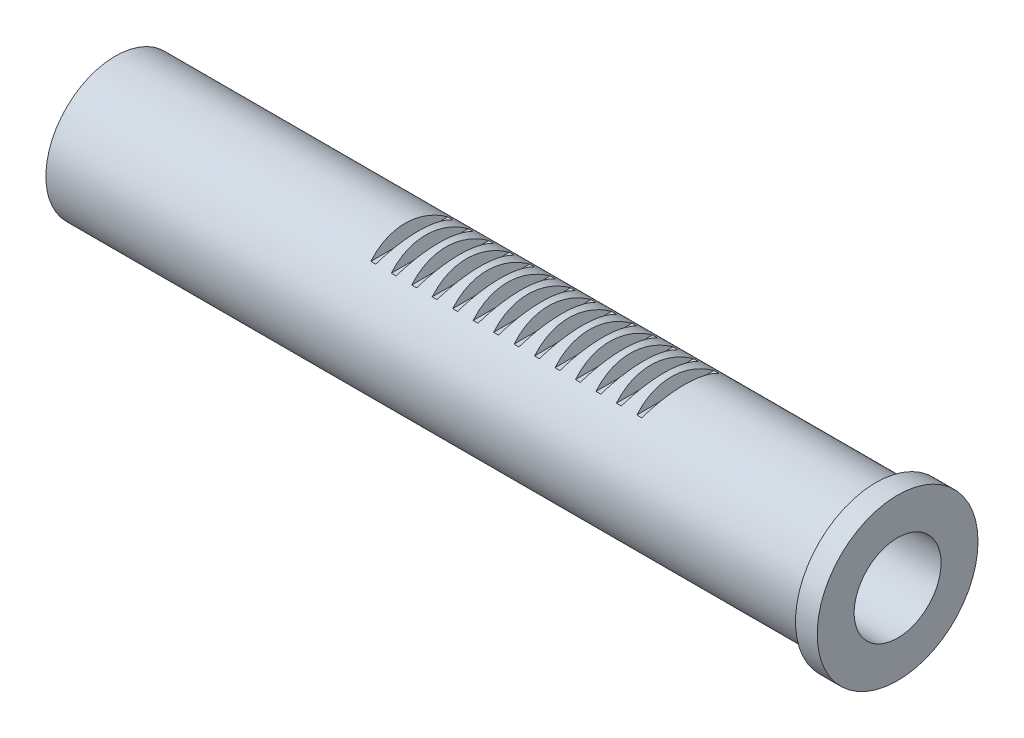
SolidWorks part; units mm, degrees
ref_plane "Front Plane" through (0, 0, 0) normal (0, 0, 1) x (1, 0, 0)
ref_plane "Top Plane" through (0, 0, 0) normal (0, 1, 0) x (1, 0, 0)
ref_plane "Right Plane" through (0, 0, 0) normal (1, 0, 0) x (0, 0, -1)
other "Configuration Table"
sketch "Sketch1" plane through (0, 0, 0) normal (1, 0, 0) x (0, 0, -1)
  circle A0 centre (0, 0) radius 16
  dimension "D1" = 32
extrude "Boss-Extrude1" add sketch "Sketch1" along normal blind 175
sketch "Sketch2" plane through (175, 0, 0) normal (1, 0, 0) x (0, 0, -1)
  circle A0 centre (0, 0) radius 18.5
  dimension "D1" = 37
extrude "Boss-Extrude2" add sketch "Sketch2" along normal blind 5
sketch "Sketch3" plane through (180, 0, 0) normal (1, 0, 0) x (0, 0, -1)
  circle A0 centre (0, 0) radius 10
  dimension "D1" = 20
extrude "Cut-Extrude1" cut sketch "Sketch3" against normal blind 100
sketch "Sketch4" plane through (180, 0, 0) normal (1, 0, 0) x (0, 0, -1)
  circle A0 centre (0, 0) radius 6
  dimension "D1" = 12
extrude "Cut-Extrude2" cut sketch "Sketch4" against normal blind 8000
sketch "Sketch5" plane through (0, 0, 0) normal (0, 0, 1) x (1, 0, 0)
  line L0 (0, 0) -> (50, 0)
  line L1 (0, 6) -> (0, -6) construction
  line L2 (50, 0) -> (50, 6)
  line L3 (50, 6) -> (0, 11)
  line L4 (0, 16) -> (0, -16) construction
  line L5 (0, 11) -> (0, 0)
  line L6 (50, 6) -> (47, 6) construction
  line L7 (47, 6) -> (47, 6.3) construction
  line L8 (80, -6) -> (80, 6) construction
  dimension "D1" = 6
  dimension "D2" = 3
  dimension "D3" = 0.3
  dimension "D4" = 30
revolve "Cut-Revolve1" cut sketch "Sketch5" angle 360 about L0
sketch "Sketch6" plane through (0, 0, 0) normal (0, 0, 1) x (1, 0, 0)
  line L0 (0, 0) -> (68.2, 0) construction
  line L1 (68.2, 0) -> (68.2, 41.9266) construction
  line L2 (69.9952, 16.6972) -> (66.4048, 16.6972)
  line L3 (66.4048, 16.6972) -> (67.635, 13.3172)
  line L4 (67.635, 13.3172) -> (68.765, 13.3172)
  line L5 (67.0225, 15) -> (69.3775, 15) construction
  line L6 (180, -18.5) -> (180, 18.5) construction
  line L7 (69.9952, 16.6972) -> (68.765, 13.3172)
  line L8 (72.345, 13.3172) -> (73.475, 13.3172)
  line L9 (74.7052, 16.6972) -> (73.475, 13.3172)
  line L10 (74.7052, 16.6972) -> (71.1148, 16.6972)
  line L11 (71.1148, 16.6972) -> (72.345, 13.3172)
  line L12 (77.055, 13.3172) -> (78.185, 13.3172)
  line L13 (79.4152, 16.6972) -> (78.185, 13.3172)
  line L14 (79.4152, 16.6972) -> (75.8248, 16.6972)
  line L15 (75.8248, 16.6972) -> (77.055, 13.3172)
  line L16 (81.765, 13.3172) -> (82.895, 13.3172)
  line L17 (84.1252, 16.6972) -> (82.895, 13.3172)
  line L18 (84.1252, 16.6972) -> (80.5348, 16.6972)
  line L19 (80.5348, 16.6972) -> (81.765, 13.3172)
  line L20 (86.475, 13.3172) -> (87.605, 13.3172)
  line L21 (88.8352, 16.6972) -> (87.605, 13.3172)
  line L22 (88.8352, 16.6972) -> (85.2448, 16.6972)
  line L23 (85.2448, 16.6972) -> (86.475, 13.3172)
  line L24 (91.185, 13.3172) -> (92.315, 13.3172)
  line L25 (93.5452, 16.6972) -> (92.315, 13.3172)
  line L26 (93.5452, 16.6972) -> (89.9548, 16.6972)
  line L27 (89.9548, 16.6972) -> (91.185, 13.3172)
  line L28 (95.895, 13.3172) -> (97.025, 13.3172)
  line L29 (98.2552, 16.6972) -> (97.025, 13.3172)
  line L30 (98.2552, 16.6972) -> (94.6648, 16.6972)
  line L31 (94.6648, 16.6972) -> (95.895, 13.3172)
  line L32 (100.605, 13.3172) -> (101.735, 13.3172)
  line L33 (102.9652, 16.6972) -> (101.735, 13.3172)
  line L34 (102.9652, 16.6972) -> (99.3748, 16.6972)
  line L35 (99.3748, 16.6972) -> (100.605, 13.3172)
  line L36 (105.315, 13.3172) -> (106.445, 13.3172)
  line L37 (107.6752, 16.6972) -> (106.445, 13.3172)
  line L38 (107.6752, 16.6972) -> (104.0848, 16.6972)
  line L39 (104.0848, 16.6972) -> (105.315, 13.3172)
  line L40 (110.025, 13.3172) -> (111.155, 13.3172)
  line L41 (112.3852, 16.6972) -> (111.155, 13.3172)
  line L42 (112.3852, 16.6972) -> (108.7948, 16.6972)
  line L43 (108.7948, 16.6972) -> (110.025, 13.3172)
  line L44 (114.735, 13.3172) -> (115.865, 13.3172)
  line L45 (117.0952, 16.6972) -> (115.865, 13.3172)
  line L46 (117.0952, 16.6972) -> (113.5048, 16.6972)
  line L47 (113.5048, 16.6972) -> (114.735, 13.3172)
  line L48 (119.445, 13.3172) -> (120.575, 13.3172)
  line L49 (121.8052, 16.6972) -> (120.575, 13.3172)
  line L50 (121.8052, 16.6972) -> (118.2148, 16.6972)
  line L51 (118.2148, 16.6972) -> (119.445, 13.3172)
  line L52 (124.155, 13.3172) -> (125.285, 13.3172)
  line L53 (126.5152, 16.6972) -> (125.285, 13.3172)
  line L54 (126.5152, 16.6972) -> (122.9248, 16.6972)
  line L55 (122.9248, 16.6972) -> (124.155, 13.3172)
  line L56 (128.865, 13.3172) -> (129.995, 13.3172)
  line L57 (131.2252, 16.6972) -> (129.995, 13.3172)
  line L58 (131.2252, 16.6972) -> (127.6348, 16.6972)
  line L59 (127.6348, 16.6972) -> (128.865, 13.3172)
  point P13 (68.2, 15)
  point P14 (68.2, 13.3172)
  point P15 (68.2, 16.6972)
  dimension "D1" = 20
  dimension "D2" = 3.38
  dimension "D3" = 1.13
  dimension "D4" = 2.355
  dimension "D5" = 111.8
  dimension "D6" = 15
  dimension "D7" = 14
extrude "Cut-Extrude3" cut sketch "Sketch6" against normal through all both and the other way through all
